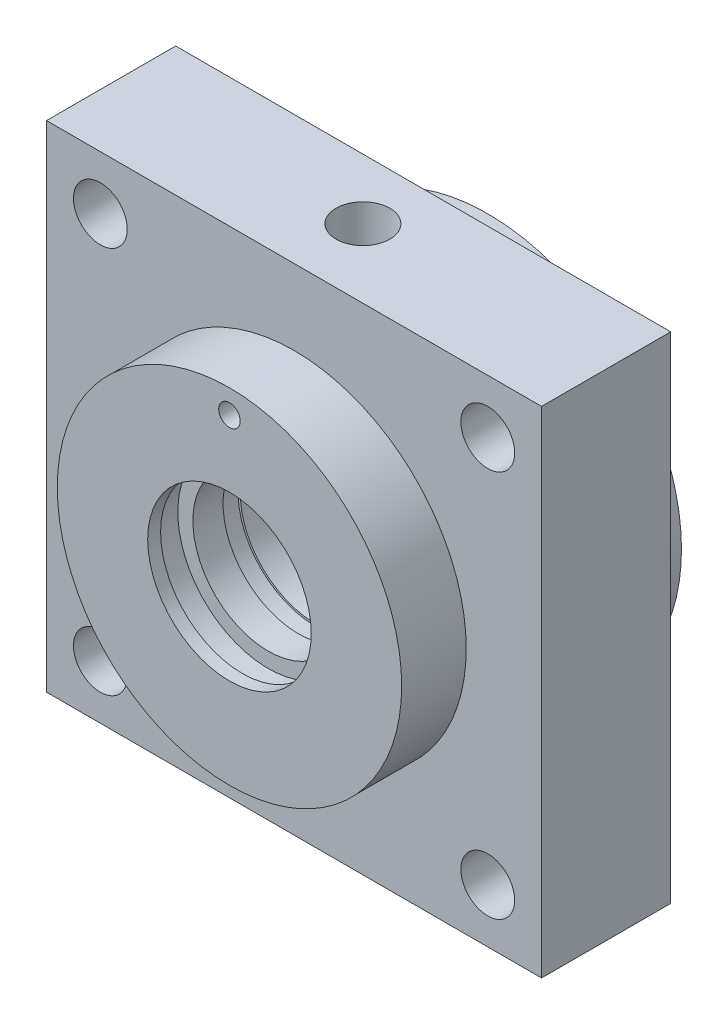
from build123d import *

# Parameters (mm, degrees)
SKETCH_1_W          = 115
SKETCH_1_H          = 115
SKETCH_1_R          = 6.25
EXTRUDE_1_DEPTH     = 30
SKETCH_2_R          = 40
EXTRUDE_2_DEPTH     = 15
SKETCH_22_R         = 45
EXTRUDE_4_DEPTH     = 15
SKETCH_23_W         = 6.5
SKETCH_23_H         = 5
SKETCH_24_R         = 2.5
CUT_EXTRUDE_5_DEPTH = 30
SKETCH_28_R         = 3
CUT_EXTRUDE_6_DEPTH = 25


with BuildPart() as part:
    # 草图1 → 凸台-拉伸1 (new body)
    with BuildSketch(Plane.XY):
        Rectangle(SKETCH_1_W, SKETCH_1_H)
        with Locations((-45, 45)):
            Circle(SKETCH_1_R, mode=Mode.SUBTRACT)
        with Locations((45, 45)):
            Circle(SKETCH_1_R, mode=Mode.SUBTRACT)
        with Locations((45, -45)):
            Circle(SKETCH_1_R, mode=Mode.SUBTRACT)
        with Locations((-45, -45)):
            Circle(SKETCH_1_R, mode=Mode.SUBTRACT)
    extrude(amount=EXTRUDE_1_DEPTH)

    # 草图2 → 凸台-拉伸2 (add)
    with BuildSketch(Plane.XY.offset(30)):
        Circle(SKETCH_2_R)
    extrude(amount=EXTRUDE_2_DEPTH)

    # 草图22 → 凸台-拉伸4 (add)
    with BuildSketch(Plane(origin=(0, 0, 0), x_dir=(-1, 0, 0), z_dir=(0, 0, -1))):
        Circle(SKETCH_22_R)
    extrude(amount=EXTRUDE_4_DEPTH)

    # 草图23 → 切除-旋转2 (revolve, cut)
    with BuildSketch(Plane(origin=(0, 0, 0), x_dir=(0, 0, -1), z_dir=(1, 0, 0)), mode=Mode.PRIVATE) as cut_revolve_2_sk:
        Polygon((-45, 19), (-42, 19), (-42, 21), (-36, 21), (-36, 17.5), (-29, 17.5), (-29, 18), (-25, 18), (-25, 17.5), (-18, 17.5), (-18, 18), (-14, 18), (-14, 17.5), (-8, 17.5), (-8, 18), (-1.5, 18), (-1.5, 17.5), (5.5, 17.5), (5.5, 20), (12, 20), (12, 19), (15, 19), (15, 0), (-45, 0), align=None)
        with Locations((8.25, 42.5)):
            Rectangle(SKETCH_23_W, SKETCH_23_H)
    revolve(cut_revolve_2_sk.sketch.rotate(Axis((0, 0, 45), (0, 0, -1)), 90), axis=Axis((0, 0, 45), (0, 0, -1)), mode=Mode.SUBTRACT)

    # 草图24 → 切除-拉伸5 (cut)
    with BuildSketch(Plane.XY.offset(45)):
        with Locations((0, 34.5)):
            Circle(SKETCH_24_R)
    extrude(amount=-CUT_EXTRUDE_5_DEPTH, mode=Mode.SUBTRACT)

    # 草图26 → 1/4 NPT 螺纹孔2 (revolve, cut)
    with BuildSketch(Plane(origin=(0, 57.5, 14), x_dir=(0, 0, 1), z_dir=(1, 0, 0))):
        Polygon((0, 0), (0, 20.412347279), (5.5626, 17.07), (5.5626, 10.02), (5.943676082, 10.02), (6.2436883, 0), align=None)
    revolve(axis=Axis((0, 63.85, 14), (0, -1, 0)), mode=Mode.SUBTRACT)

    # 草图28 → 切除-拉伸6 (cut)
    with BuildSketch(Plane(origin=(0, 57.5, 0), x_dir=(1, 0, 0), z_dir=(0, 1, 0))):
        with Locations(Location((0, -14, 0), (0, 0, 270))):
            Circle(SKETCH_28_R)
    extrude(amount=-CUT_EXTRUDE_6_DEPTH, mode=Mode.SUBTRACT)


solid = part.part
